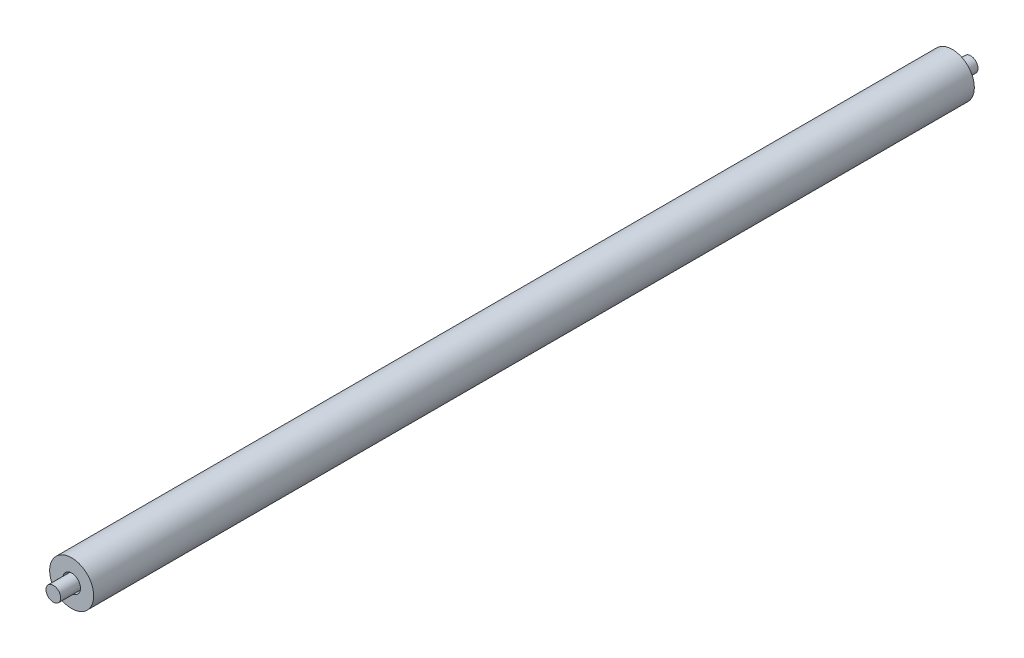
from build123d import *

# Parameters (mm, degrees)
SKETCH_1_R          = 10
EXTRUDE_1_DEPTH     = 625
SKETCH_2_R          = 30
SKETCH_2_R_2        = 10
EXTRUDE_2_DEPTH     = 600
SKETCH_3_R          = 12
SKETCH_3_R_2        = 5
CUT_EXTRUDE_1_DEPTH = 10


with BuildPart() as part:
    # 草图1 → 凸台-拉伸1 (new, symmetric)
    with BuildSketch(Plane.XY):
        Circle(SKETCH_1_R)
    extrude(amount=EXTRUDE_1_DEPTH, both=True)


with BuildPart() as body_2:
    # 草图2 → 凸台-拉伸2 (new, symmetric)
    with BuildSketch(Plane.XY):
        Circle(SKETCH_2_R)
        Circle(SKETCH_2_R_2, mode=Mode.SUBTRACT)
    extrude(amount=EXTRUDE_2_DEPTH, both=True)

    # 草图3 → 切除-拉伸1 (cut)
    with BuildSketch(Plane.XY.offset(600)):
        Circle(SKETCH_3_R)
        Circle(SKETCH_3_R_2, mode=Mode.SUBTRACT)
    cut_extrude_1 = extrude(amount=-CUT_EXTRUDE_1_DEPTH, mode=Mode.SUBTRACT)

    # 镜向1: 切除-拉伸1 across plane
    add(cut_extrude_1.mirror(Plane.XY), mode=Mode.SUBTRACT)


solid = Compound([part.part, body_2.part])
